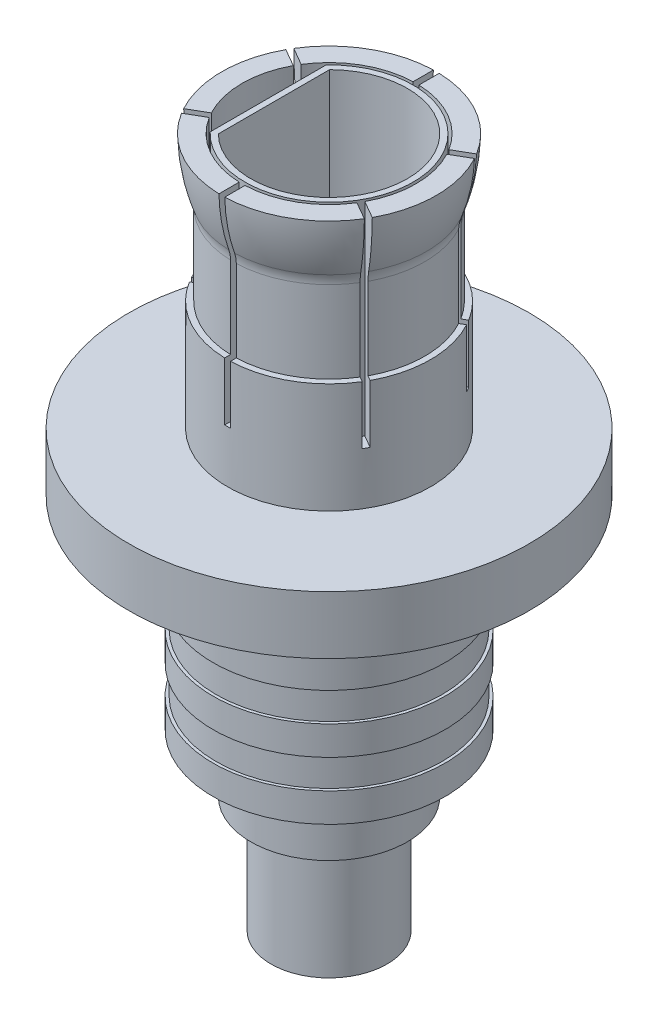
SolidWorks part; units mm, degrees
material "铜"
ref_plane "Front Plane" through (0, 0, 0) normal (0, 0, 1) x (1, 0, 0)
ref_plane "Top Plane" through (0, 0, 0) normal (0, 1, 0) x (1, 0, 0)
ref_plane "Right Plane" through (0, 0, 0) normal (1, 0, 0) x (0, 0, -1)
sketch "Sketch1" plane through (0, 0, 0) normal (0, 0, 1) x (1, 0, 0)
  line L0 (0, 0) -> (0, 19.6522) construction
  line L1 (-1.35, 0) -> (-1.35, 1)
  line L2 (-1.35, 1) -> (-2, 1)
  line L3 (-2, 1) -> (-2, 1.5)
  line L4 (-2, 4.5) -> (-3.45, 4.5)
  line L5 (-1.65, 7.4) -> (-1.65, 8.8108)
  line L6 (-1.35, 0) -> (-1, 0)
  line L7 (-1.65, 7.4) -> (-1.75, 7.4)
  line L8 (-1.849, 9.9) -> (-1.5, 9.9)
  line L9 (-1.5, 9.9) -> (-1.5, 3.9)
  line L10 (-1.75, 7.4) -> (-1.75, 5.5)
  line L11 (-1.75, 5.5) -> (-3.45, 5.5)
  line L12 (-3.45, 5.5) -> (-3.45, 4.5)
  line L13 (-0.6, -2) -> (-0.6, 3.9)
  line L14 (-0.6, 3.9) -> (-1.5, 3.9)
  line L15 (-2, 2) -> (-1.95, 2)
  line L16 (-1.95, 2) -> (-1.95, 1.5)
  line L17 (-1.95, 1.5) -> (-2, 1.5)
  line L18 (-2, 3) -> (-1.95, 3)
  line L19 (-1.95, 3) -> (-1.95, 2.5)
  line L20 (-1.95, 2.5) -> (-2, 2.5)
  line L24 (-1.95, 4) -> (-1.95, 3.5)
  line L25 (-2, 4) -> (-1.95, 4)
  line L26 (-1.95, 3.5) -> (-2, 3.5)
  line L27 (-2, 4) -> (-2, 4.5)
  line L28 (-2, 3) -> (-2, 3.5)
  line L30 (-2, 2) -> (-2, 2.5)
  line L31 (0, 0) -> (5.1651, 0) construction
  line L32 (-1, 0) -> (-1, -2)
  line L33 (-1, -2) -> (-0.6, -2)
  arc A0 (-1.849, 9.9) -> (-1.6786, 8.9774) centre (1.15, 9.977) ccw
  arc A1 (-1.65, 8.8108) -> (-1.6786, 8.9774) centre (-2.15, 8.8108) ccw
  point P37 (-1.65, 8.9)
  dimension "D7" = 3.3
  dimension "D6" = 3.7
  dimension "D16" = 3
  dimension "D21" = 0.5
  dimension "D1" = 2.7
  dimension "D2" = 1
  dimension "D3" = 0.5
  dimension "D4" = 4
  dimension "D5" = 3.5
  dimension "D8" = 1.9
  dimension "D9" = 1
  dimension "D10" = 1.5
  dimension "D11" = 3
  dimension "D12" = 1.2
  dimension "D13" = 6
  dimension "D14" = 1
  dimension "D15" = 6.9
  dimension "D17" = 0.5
  dimension "D18" = 0.5
  dimension "D19" = 0.5
  dimension "D20" = 3.9
  dimension "D22" = 0.5
  dimension "D23" = 0.5
  dimension "D24" = 2
  dimension "D25" = 2
  dimension "D26" = 0.5
revolve "Revolve1" add sketch "Sketch1" angle 360 about L0
sketch "Sketch2" plane through (0, 9.9, 0) normal (0, 1, 0) x (1, 0, 0)
  line L1 (-0.05, -2.2683) -> (0.05, -2.2683)
  line L2 (-0.05, -2.2683) -> (-0.05, 2.2683)
  line L3 (-0.05, 2.2683) -> (0.05, 2.2683)
  line L4 (0.05, -2.2683) -> (0.05, 2.2683)
  line L5 (-0.05, -2.2683) -> (0.05, 2.2683) construction
  line L6 (-0.05, 2.2683) -> (0.05, -2.2683) construction
  point P0 (0, 0)
  dimension "D1" = 0.1
extrude "Cut-Extrude1" cut sketch "Sketch2" against normal blind 3.5
pattern_circular "CirPattern1" count 3 over 360 about axis through (0, 0, 0) along (0, 1, 0) of "Cut-Extrude1"
sketch "Sketch3" plane through (0, 0, 0) normal (0, -1, 0) x (1, 0, 0)
  circle A0 centre (0, 0) radius 1.35
sketch "Sketch5" plane through (0, 3.9, 0) normal (0, 1, 0) x (1, 0, 0)
  line L0 (-1.05, 1) -> (-1.05, -1)
  arc A1 (-1.05, -1) -> (-1.05, 1) centre (0, 0) ccw
  dimension "D1" = 2.9
  dimension "D2" = 2
extrude "Boss-Extrude1" add sketch "Sketch5" along normal blind 6
sketch "Sketch6" plane through (0, 9.9, 0) normal (0, 1, 0) x (1, 0, 0)
  line L2 (-0.95, 0.9592) -> (-0.95, -0.9592)
  line L3 (-0.95, 0.9592) -> (-0.95, -0.9592)
  arc A3 (-0.95, -0.9592) -> (-0.95, 0.9592) centre (0, 0) ccw
  arc A4 (-0.95, -0.9592) -> (-0.95, 0.9592) centre (0, 0) ccw
  dimension "D1" = 0.1
extrude "Cut-Extrude2" cut sketch "Sketch6" against normal blind 5.9
sketch "Sketch7" plane through (0, 4, 0) normal (0, 1, 0) x (1, 0, 0)
  circle A0 centre (0, 0) radius 0.565
  dimension "D1" = 1.13
extrude "Cut-Extrude3" cut sketch "Sketch7" against normal blind 2
